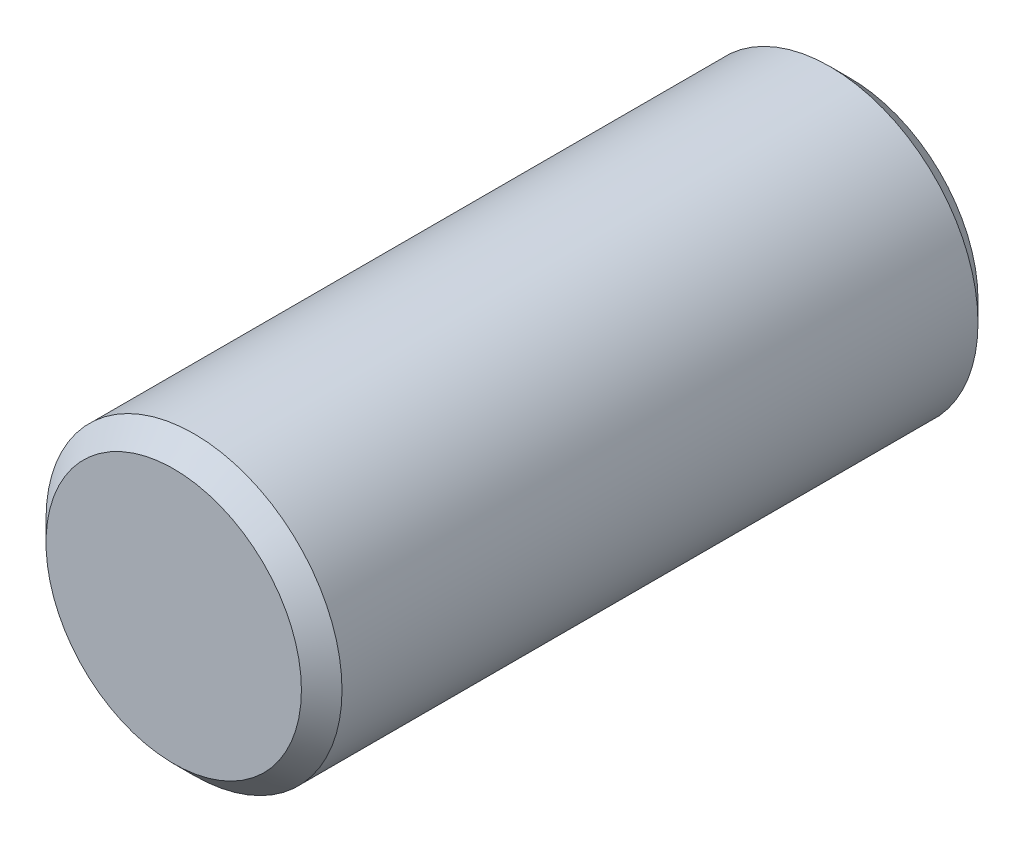
SolidWorks part; units mm, degrees
material "20"
ref_plane "Front plane" through (0, 0, 0) normal (0, 0, 1) x (1, 0, 0)
ref_plane "Top plane" through (0, 0, 0) normal (0, 1, 0) x (1, 0, 0)
ref_plane "Right plane" through (0, 0, 0) normal (1, 0, 0) x (0, 0, -1)
sketch "Sketch1" plane through (0, 0, 0) normal (0, 0, 1) x (1, 0, 0)
  circle A0 centre (0, 0) radius 11.1125
  dimension "D1" = 22.225
extrude "Extrude1" add sketch "Sketch1" along normal mid plane 50.8
chamfer "Chamfer1" distance 1.524 angle 45 2 edges at (11.1125, 0, 25.4) (11.1125, 0, -25.4)
